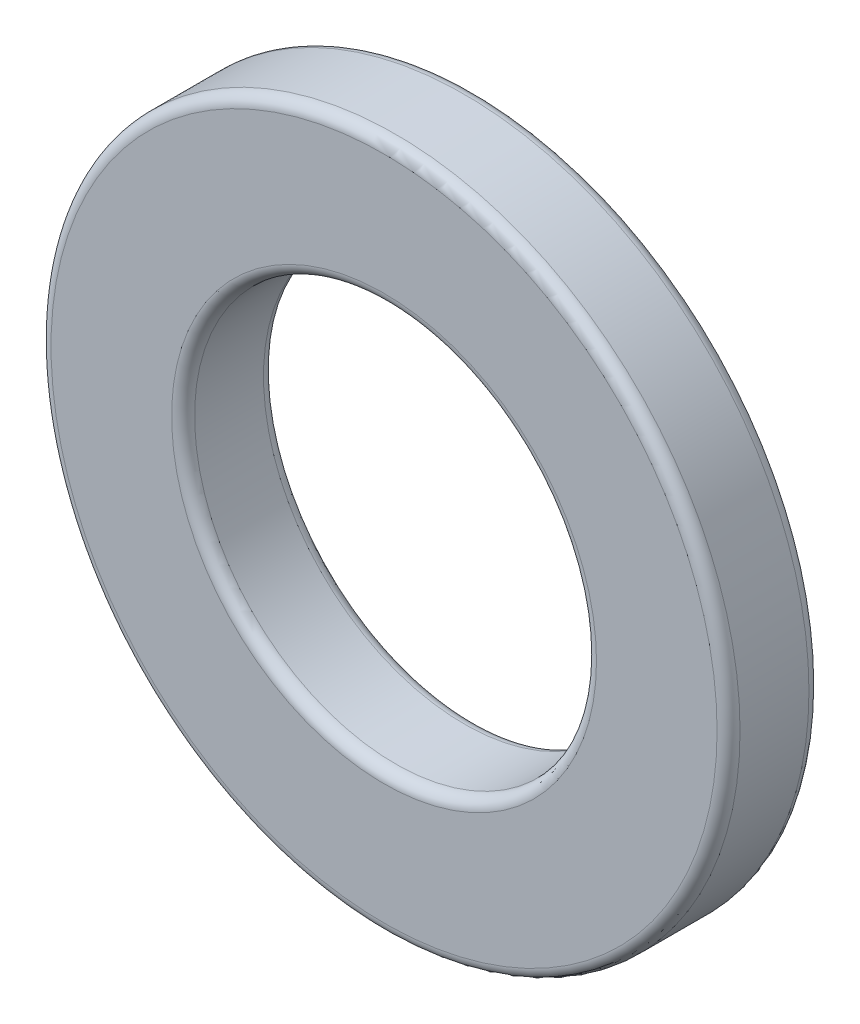
SolidWorks part; units mm, degrees
material "标准件"
ref_plane "前视基准面" through (0, 0, 0) normal (0, 0, 1) x (1, 0, 0)
ref_plane "上视基准面" through (0, 0, 0) normal (0, 1, 0) x (1, 0, 0)
ref_plane "右视基准面" through (0, 0, 0) normal (1, 0, 0) x (0, 0, -1)
sketch "草图1" plane through (0, 0, 0) normal (0, 0, 1) x (1, 0, 0)
  circle A0 centre (0, 0) radius 17.5
  circle A1 centre (0, 0) radius 30
  dimension "D1" = 35
  dimension "D2" = 60
extrude "凸台-拉伸1" add sketch "草图1" along normal blind 8
fillet "圆角1" radius 1 4 edges at (17.5, 0, 0) (17.5, 0, 8) (30, 0, 0) (30, 0, 8)
